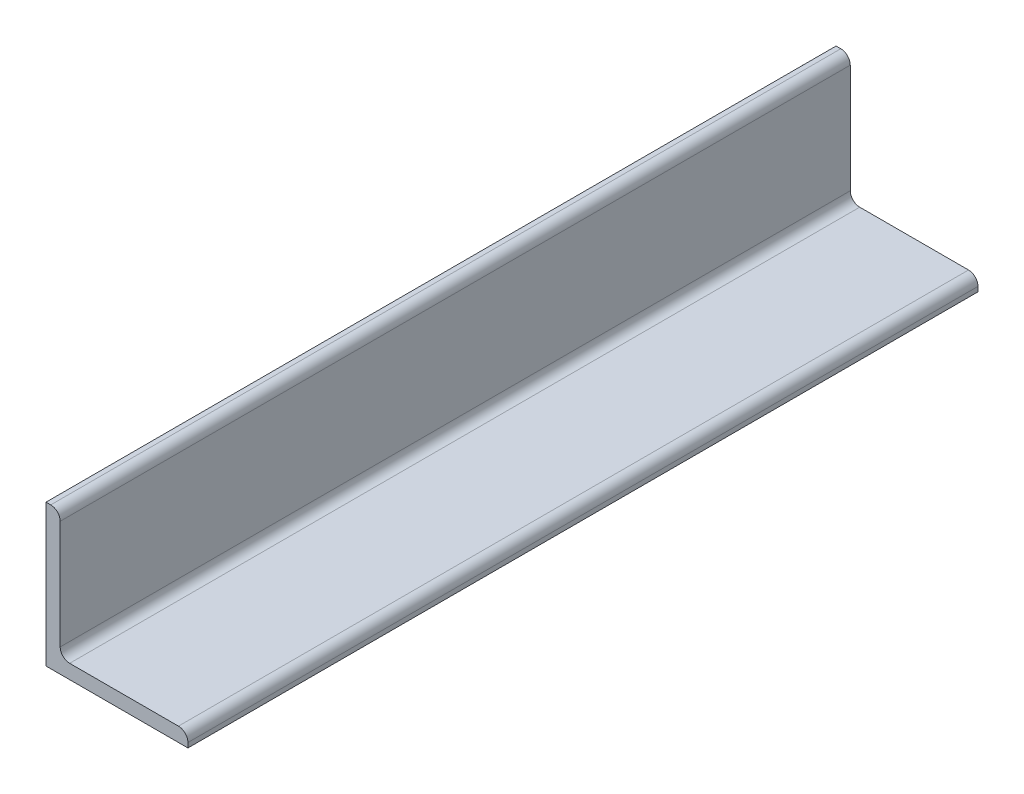
SolidWorks part; units mm, degrees
material "Plain Carbon Steel"
ref_plane "Front Plane" through (0, 0, 0) normal (0, 0, 1) x (1, 0, 0)
ref_plane "Top Plane" through (0, 0, 0) normal (0, 1, 0) x (1, 0, 0)
ref_plane "Right Plane" through (0, 0, 0) normal (1, 0, 0) x (0, 0, -1)
sketch "Sketch1" plane through (0, 0, 0) normal (0, 0, 1) x (1, 0, 0)
  line L0 (0, 0) -> (30, 0)
  line L1 (0, 0) -> (0, 30)
  line L2 (5, 3) -> (28, 3)
  line L3 (3, 5) -> (3, 28)
  line L4 (0, 30) -> (1, 30)
  line L5 (30, 1) -> (30, 0)
  line L6 (3, 3) -> (3, 30) construction
  line L7 (3, 3) -> (30, 3) construction
  arc A0 (1, 30) -> (3, 28) centre (1, 28) cw
  arc A1 (5, 3) -> (3, 5) centre (5, 5) cw
  arc A2 (30, 1) -> (28, 3) centre (28, 1) ccw
  dimension "D3" = 2
  dimension "D1" = 30
  dimension "D2" = 3
extrude "Boss-Extrude1" add sketch "Sketch1" along normal blind 167
